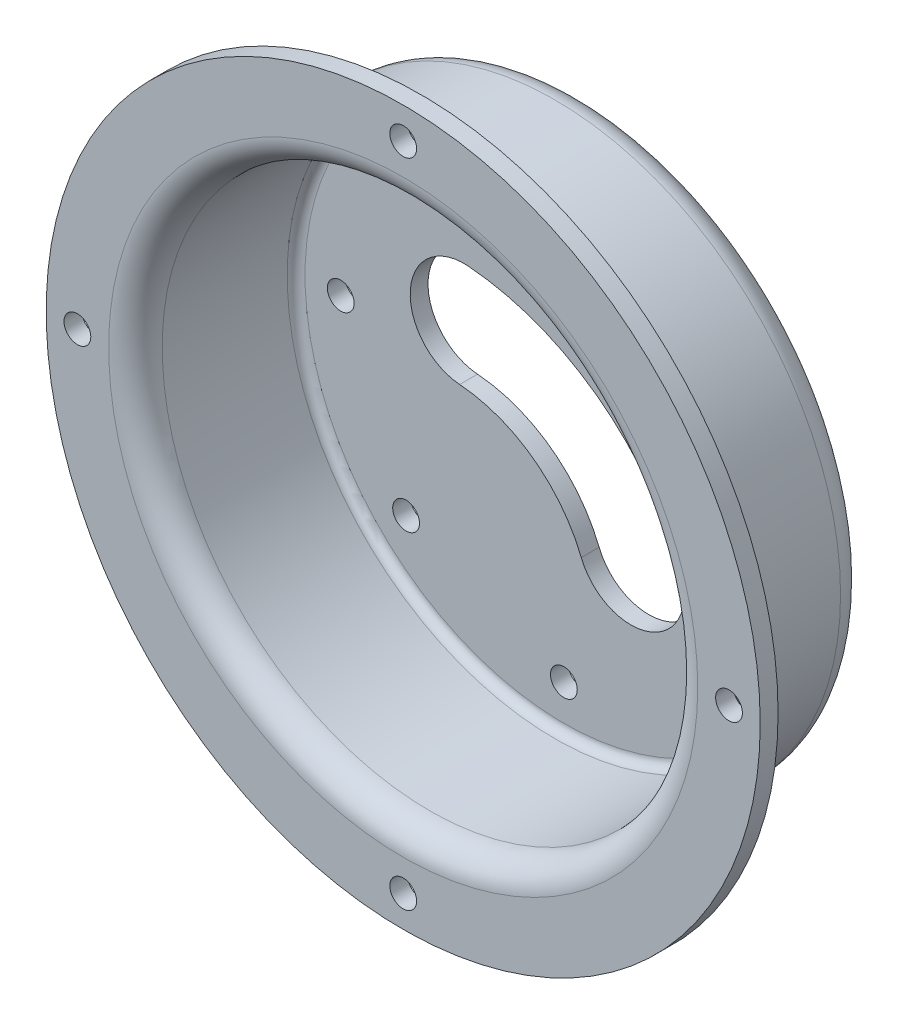
SolidWorks part; units mm, degrees
ref_plane "Front Plane" through (0, 0, 0) normal (0, 0, 1) x (1, 0, 0)
ref_plane "Top Plane" through (0, 0, 0) normal (0, 1, 0) x (1, 0, 0)
ref_plane "Right Plane" through (0, 0, 0) normal (1, 0, 0) x (0, 0, -1)
other "Configuration Table"
sketch "Sketch1" plane through (0, 0, 0) normal (0, 0, 1) x (1, 0, 0)
  circle A0 centre (0, 0) radius 160
  circle A2 centre (0, 0) radius 125 construction
  circle A3 centre (0, 125) radius 7.5
  circle A4 centre (88.3883, 88.3883) radius 7.5
  circle A5 centre (125, 0) radius 7.5
  circle A6 centre (88.3883, -88.3883) radius 7.5
  circle A7 centre (0, -125) radius 7.5
  circle A8 centre (-88.3883, -88.3883) radius 7.5
  circle A9 centre (-125, 0) radius 7.5
  circle A10 centre (-88.3883, 88.3883) radius 7.5
  arc A14 (-53.8031, 50.0377) -> (-58.3711, -9.7881) centre (-56.0871, 20.1248) ccw
  arc A15 (9.7519, -59.6843) -> (65.4122, -37.2806) centre (37.5821, -48.4825) ccw
  arc A19 (9.7519, -59.6843) -> (-58.3711, -9.7881) centre (-64.4619, -89.5559) ccw
  arc A20 (44.8843, -77.5802) -> (-86.0321, 18.3085) centre (-64.4619, -89.5559) ccw construction
  arc A21 (65.4122, -37.2806) -> (-53.8031, 50.0377) centre (-64.4619, -89.5559) ccw
  point P24 (0, 0)
  dimension "D1" = 320
  dimension "D3" = 250
  dimension "D4" = 15
  dimension "D5" = 8
extrude "Boss-Extrude1" add sketch "Sketch1" along normal blind 10
sketch "Sketch2" plane through (0, 0, 10) normal (0, 0, 1) x (1, 0, 0)
  circle A0 centre (0, 0) radius 160
  circle A1 centre (0, 0) radius 150
  dimension "D1" = 300
extrude "Boss-Extrude2" add sketch "Sketch2" along normal blind 80
sketch "Sketch3" plane through (0, 0, 90) normal (0, 0, 1) x (1, 0, 0)
  circle A0 centre (0, 0) radius 150
  circle A1 centre (0, 0) radius 200
  circle A2 centre (0, 0) radius 182.5 construction
  circle A3 centre (0, 182.5) radius 7.5
  circle A9 centre (182.5, 0) radius 7.5
  circle A10 centre (0, -182.5) radius 7.5
  circle A11 centre (-182.5, 0) radius 7.5
  point P14 (0, 0)
  point P16 (0, 0)
  point P18 (0, 0)
  dimension "D1" = 400
  dimension "D2" = 15
  dimension "D3" = 365
  dimension "D4" = 4
extrude "Boss-Extrude3" add sketch "Sketch3" along normal blind 10
fillet "Fillet1" radius 5 2 edges at (160, 0, 90) (150, 0, 10)
fillet "Fillet2" radius 15 2 edges at (150, 0, 100) (160, 0, 0)
